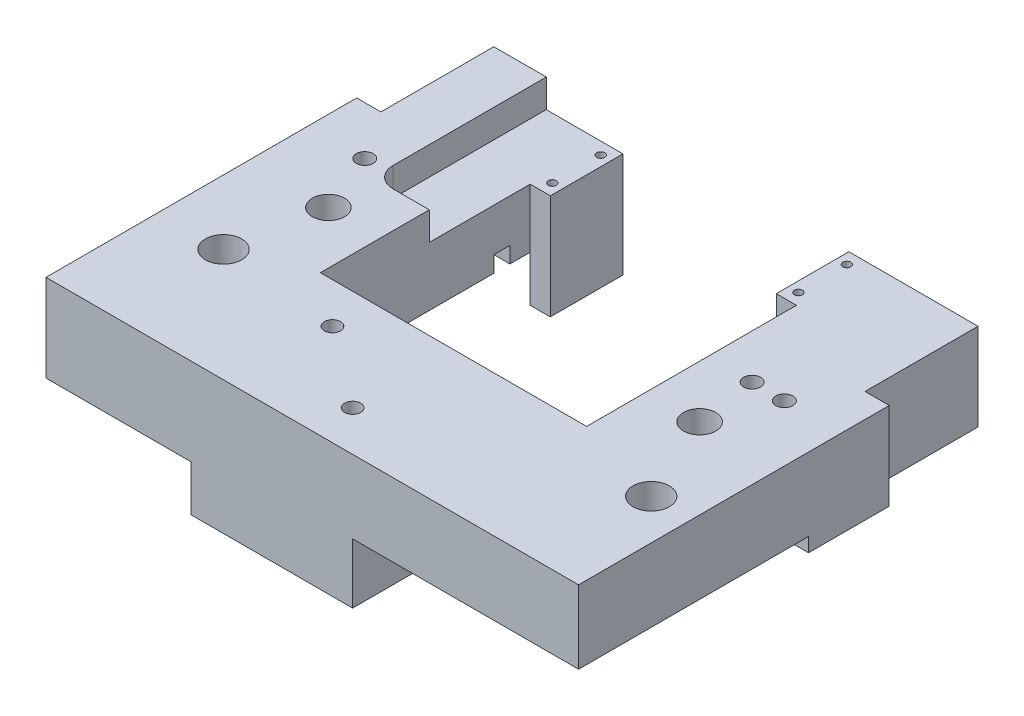
SolidWorks part; units mm, degrees
ref_plane "前视基准面" through (0, 0, 0) normal (0, 0, 1) x (1, 0, 0)
ref_plane "上视基准面" through (0, 0, 0) normal (0, 1, 0) x (1, 0, 0)
ref_plane "右视基准面" through (0, 0, 0) normal (1, 0, 0) x (0, 0, -1)
sketch "草图1" plane through (0, 0, 0) normal (0, 0, 1) x (1, 0, 0)
  line L1 (-76.0678, 7.6907) -> (55.9322, 7.6907)
  line L2 (-76.0678, 7.6907) -> (-76.0678, -25.3093)
  line L3 (-76.0678, -25.3093) -> (55.9322, -25.3093)
  line L4 (55.9322, 7.6907) -> (55.9322, -25.3093)
  dimension "D1" = 132
  dimension "D2" = 33
extrude "凸台-拉伸1" add sketch "草图1" along normal blind 105
sketch "草图2" plane through (0, 7.6907, 0) normal (0, 1, 0) x (1, 0, 0)
  line L0 (-43.0678, -70) -> (22.9322, -70)
  line L1 (22.9322, -70) -> (22.9322, -18)
  line L2 (22.9322, -18) -> (17.9322, -18)
  line L3 (17.9322, -18) -> (17.9322, 0)
  line L4 (55.9322, 0) -> (-76.0678, 0) construction
  line L5 (-43.0678, -70) -> (-43.0678, -18)
  line L6 (-43.0678, -18) -> (-38.0678, -18)
  line L7 (-38.0678, -18) -> (-38.0678, 0)
  line L8 (-38.0678, 0) -> (17.9322, 0)
  line L9 (55.9322, -105) -> (-76.0678, -105) construction
  line L10 (-76.0678, -105) -> (-76.0678, 0) construction
  line L11 (55.9322, -105) -> (55.9322, 0) construction
  dimension "D1" = 35
  dimension "D2" = 33
  dimension "D3" = 33
  dimension "D4" = 52
  dimension "D5" = 52
  dimension "D6" = 5
  dimension "D7" = 5
extrude "切除-拉伸1" cut sketch "草图2" against normal up to next
sketch "草图3" plane through (0, -25.3093, 0) normal (0, -1, 0) x (1, 0, 0)
  line L9 (-0.0678, 70) -> (-0.0678, 105)
  line L12 (55.9322, 105) -> (55.9322, 28)
  line L13 (55.9322, 105) -> (55.9322, 0) construction
  line L14 (55.9322, 28) -> (49.9322, 28)
  line L15 (55.9322, 105) -> (-0.0678, 105)
  line L16 (-0.0678, 70) -> (22.9322, 70)
  line L17 (22.9322, 70) -> (22.9322, 0)
  line L20 (49.9322, 28) -> (49.9322, 0)
  line L21 (17.9322, 0) -> (55.9322, 0) construction
  line L22 (49.9322, 0) -> (22.9322, 0)
  line L23 (-40.0678, 105) -> (-40.0678, 70)
  line L26 (-40.0678, 70) -> (-43.0678, 70)
  line L27 (-43.0678, 70) -> (-43.0678, 0)
  line L28 (-76.0678, 0) -> (-38.0678, 0) construction
  line L29 (-43.0678, 0) -> (-70.0678, 0)
  line L30 (-70.0678, 0) -> (-70.0678, 28)
  line L31 (-70.0678, 28) -> (-76.0678, 28)
  line L32 (-76.0678, 28) -> (-76.0678, 105)
  line L33 (-76.0678, 105) -> (-40.0678, 105)
  dimension "D1" = 56
  dimension "D2" = 6
  dimension "D3" = 77
  dimension "D4" = 23
  dimension "D5" = 35
  dimension "D6" = 36
  dimension "D7" = 3
  dimension "D8" = 70
  dimension "D9" = 77
  dimension "D10" = 6
extrude "切除-拉伸2" cut sketch "草图3" against normal blind 11.37
sketch "草图4" plane through (0, -25.3093, 0) normal (0, -1, 0) x (1, 0, 0)
  line L1 (-76.0678, 28) -> (-70.0678, 28)
  line L2 (-76.0678, 28) -> (-76.0678, 0)
  line L3 (-76.0678, 0) -> (-70.0678, 0)
  line L4 (-70.0678, 28) -> (-70.0678, 0)
  line L5 (49.9322, 28) -> (55.9322, 28)
  line L6 (49.9322, 28) -> (49.9322, 0)
  line L7 (49.9322, 0) -> (55.9322, 0)
  line L8 (55.9322, 28) -> (55.9322, 0)
extrude "切除-拉伸3" cut sketch "草图4" against normal up to next
sketch "草图5" plane through (55.9322, 0, 0) normal (1, 0, 0) x (0, 0, -1)
  line L0 (-28, -13.9393) -> (-105, -13.9393) construction
  line L1 (-48, -13.9393) -> (-105, -13.9393)
  line L2 (-48, -13.9393) -> (-48, -10.4393)
  line L3 (-48, -10.4393) -> (-105, -10.4393)
  line L4 (-105, -13.9393) -> (-105, -10.4393)
  line L5 (-105, -13.9393) -> (-105, 7.6907) construction
  dimension "D1" = 3.5
  dimension "D2" = 57
extrude "切除-拉伸5" cut sketch "草图5" against normal blind 56
sketch "草图7" plane through (49.9322, 0, 0) normal (1, 0, 0) x (0, 0, -1)
  line L0 (0, -13.9393) -> (-28, -13.9393) construction
  line L1 (-23, -13.9393) -> (-27, -13.9393)
  line L2 (-23, -13.9393) -> (-23, -9.9393)
  line L3 (-23, -9.9393) -> (-27, -9.9393)
  line L4 (-27, -13.9393) -> (-27, -9.9393)
  line L5 (-28, 7.6907) -> (-28, -13.9393) construction
  dimension "D1" = 4
  dimension "D2" = 4
  dimension "D3" = 1
extrude "切除-拉伸6" cut sketch "草图7" against normal through all
sketch "草图8" plane through (0, 7.6907, 0) normal (0, 1, 0) x (1, 0, 0)
  line L0 (-38.0678, -18) -> (-43.0678, -18)
  line L1 (-43.0678, -18) -> (-43.0678, -43)
  line L2 (-43.0678, -18) -> (-43.0678, -70) construction
  line L3 (-43.0678, -43) -> (-52.0678, -43)
  line L4 (-38.0678, -18) -> (-38.0678, 0)
  line L5 (-38.0678, 0) -> (-57.0678, 0)
  line L6 (-38.0678, 0) -> (-70.0678, 0) construction
  line L7 (-57.0678, 0) -> (-57.0678, -38)
  arc A0 (-57.0678, -38) -> (-52.0678, -43) centre (-52.0678, -38) ccw
  dimension "D1" = 25
  dimension "D2" = 9
  dimension "D3" = 19
  dimension "D4" = 38
extrude "切除-拉伸7" cut sketch "草图8" against normal blind 7
sketch "草图9" plane through (0, -25.3093, 0) normal (0, -1, 0) x (1, 0, 0)
  line L0 (-76.0678, 105) -> (-76.0678, 28) construction
  line L1 (-40.0678, 105) -> (-76.0678, 105) construction
  line L2 (-43.0678, 27) -> (-43.0678, 70) construction
  line L3 (-43.0678, 70) -> (-40.0678, 70) construction
  line L4 (-70.0678, 27) -> (-43.0678, 27) construction
  line L5 (-70.0678, 28) -> (-70.0678, 27) construction
  line L6 (-43.0678, 18) -> (-38.0678, 18) construction
  line L7 (-38.0678, 18) -> (-38.0678, 0) construction
  line L8 (-43.0678, 0) -> (-38.0678, 0) construction
  line L9 (-40.0678, 105) -> (-0.0678, 105) construction
  line L10 (-0.0678, 105) -> (-0.0678, 70) construction
  line L11 (-0.0678, 70) -> (-40.0678, 70) construction
  line L12 (-40.0678, 70) -> (-40.0678, 105) construction
  line L13 (55.9322, 48) -> (55.9322, 105) construction
  line L14 (-0.0678, 105) -> (55.9322, 105) construction
  line L15 (22.9322, 48) -> (22.9322, 70) construction
  line L16 (22.9322, 70) -> (-0.0678, 70) construction
  line L17 (22.9322, 48) -> (22.9322, 27) construction
  line L18 (22.9322, 27) -> (49.9322, 27) construction
  line L19 (22.9322, 27) -> (49.9322, 27) construction
  line L20 (49.9322, 27) -> (49.9322, 28) construction
  line L21 (17.9322, 18) -> (22.9322, 18) construction
  line L22 (17.9322, 0) -> (17.9322, 18) construction
  line L23 (17.9322, 0) -> (22.9322, 0) construction
  circle A0 centre (-10.0678, 95) radius 2
  circle A1 centre (-30.0678, 80) radius 2
  circle A2 centre (-60.0678, 77) radius 4.5
  circle A3 centre (-56.0678, 55) radius 4
  circle A4 centre (-54.0678, 40) radius 2.1
  circle A5 centre (-62.0678, 40) radius 2.1
  circle A6 centre (-40.5678, 15) radius 1
  circle A7 centre (-40.5678, 3) radius 1
  circle A8 centre (45.9322, 77) radius 4.5
  circle A9 centre (35.9322, 55) radius 4
  circle A10 centre (20.4322, 15) radius 1
  circle A11 centre (20.4322, 3) radius 1
  circle A12 centre (41.9322, 40) radius 2.1
  circle A13 centre (33.9322, 40) radius 2.1
  dimension "D1" = 9
  dimension "D4" = 8
  dimension "D7" = 4.2
  dimension "D9" = 11
  dimension "D10" = 4.2
  dimension "D13" = 2
  dimension "D16" = 2
  dimension "D19" = 4
  dimension "D20" = 4
  dimension "D25" = 9
  dimension "D28" = 8
  dimension "D31" = 4.2
  dimension "D32" = 4.2
  dimension "D37" = 2
  dimension "D38" = 2
  dimension "D2" = 16
  dimension "D3" = 28
  dimension "D5" = 13
  dimension "D6" = 15
  dimension "D8" = 13
  dimension "D11" = 13
  dimension "D12" = 8
  dimension "D14" = 3
  dimension "D15" = 2.5
  dimension "D17" = 3
  dimension "D18" = 2.5
  dimension "D21" = 10
  dimension "D22" = 10
  dimension "D23" = 10
  dimension "D24" = 10
  dimension "D26" = 10
  dimension "D27" = 28
  dimension "D29" = 13
  dimension "D30" = 15
  dimension "D33" = 11
  dimension "D34" = 13
  dimension "D35" = 13
  dimension "D36" = 8
  dimension "D39" = 3
  dimension "D40" = 2.5
  dimension "D41" = 2.5
  dimension "D42" = 3
extrude "切除-拉伸8" cut sketch "草图9" against normal through all
sketch "草图10" plane through (0, -13.9393, 0) normal (0, -1, 0) x (1, 0, 0)
  circle A0 centre (-60.0678, 77) radius 7.5
  circle A1 centre (45.9322, 77) radius 7.5
  dimension "D1" = 15
  dimension "D2" = 15
extrude "切除-拉伸9" cut sketch "草图10" against normal blind 13
sketch "草图11" plane through (0, -25.3093, 0) normal (0, -1, 0) x (1, 0, 0)
  line L0 (-40.0678, 105) -> (-0.0678, 105) construction
  line L1 (-40.0678, 70) -> (-40.0678, 105) construction
  line L2 (-0.0678, 105) -> (-0.0678, 70) construction
  line L3 (-0.0678, 70) -> (-40.0678, 70) construction
  circle A0 centre (-30.0678, 95) radius 2.5
  circle A1 centre (-10.0678, 80) radius 2.5
  dimension "D5" = 5
  dimension "D6" = 5
  dimension "D1" = 10
  dimension "D2" = 10
  dimension "D3" = 10
  dimension "D4" = 10
extrude "切除-拉伸10" cut sketch "草图11" against normal blind 27
sketch "草图12" plane through (0, -10.4393, 0) normal (0, -1, 0) x (1, 0, 0)
  line L0 (-0.0678, 105) -> (55.9322, 105) construction
  line L1 (55.9322, 48) -> (55.9322, 105) construction
  circle A0 centre (34.4822, 97.6) radius 1.25
  circle A1 centre (34.4822, 71.6) radius 1.25
  dimension "D3" = 2.5
  dimension "D6" = 2.5
  dimension "D1" = 7.4
  dimension "D2" = 21.45
  dimension "D4" = 21.45
  dimension "D5" = 33.4
extrude "切除-拉伸11" cut sketch "草图12" against normal blind 8.5 contours A0 | A1
sketch "草图13" plane through (0, -13.9393, 0) normal (0, -1, 0) x (1, 0, 0)
  line L0 (-40.0678, 105) -> (-76.0678, 105) construction
  line L1 (-76.0678, 105) -> (-76.0678, 28) construction
  circle A0 centre (-68.0678, 97) radius 1.65
  dimension "D3" = 3.3
  dimension "D1" = 8
  dimension "D2" = 8
extrude "切除-拉伸12" cut sketch "草图13" against normal blind 11.5
sketch "草图16" plane through (0, -25.3093, 0) normal (0, -1, 0) x (1, 0, 0)
  line L0 (-43.0678, 0) -> (-38.0678, 0) construction
  line L1 (-38.0678, 18) -> (-38.0678, 0) construction
  line L2 (17.9322, 0) -> (22.9322, 0) construction
  line L3 (17.9322, 0) -> (17.9322, 18) construction
  circle A0 centre (-40.5678, 9) radius 1.25
  circle A1 centre (20.4322, 9) radius 1.25
  dimension "D5" = 2.5
  dimension "D6" = 2.5
  dimension "D1" = 9
  dimension "D2" = 2.5
  dimension "D3" = 9
  dimension "D4" = 2.5
extrude "切除-拉伸13" cut sketch "草图16" against normal blind 8.5
